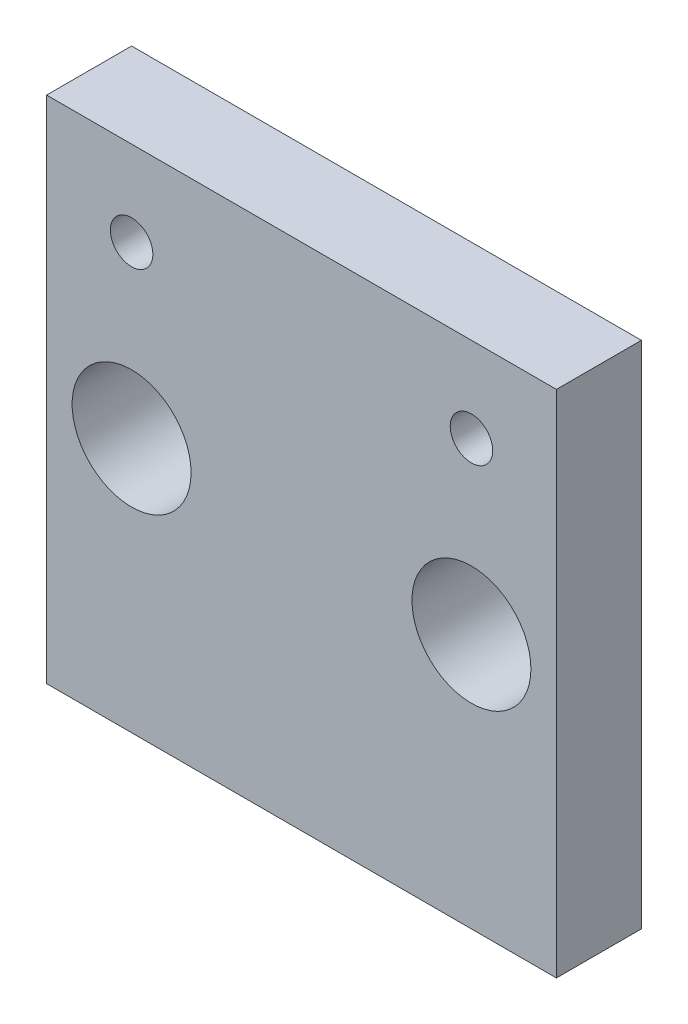
SolidWorks part; units mm, degrees
ref_plane "前视基准面" through (0, 0, 0) normal (0, 0, 1) x (1, 0, 0)
ref_plane "上视基准面" through (0, 0, 0) normal (0, 1, 0) x (1, 0, 0)
ref_plane "右视基准面" through (0, 0, 0) normal (1, 0, 0) x (0, 0, -1)
ref_plane "基准面4" through (0, 0, 5) normal (0, 0, 1) x (1, 0, 0)
sketch "草图1" plane through (0, 0, 5) normal (0, 0, 1) x (1, 0, 0)
  line L0 (-15, -15) -> (15, -15)
  line L1 (15, -15) -> (15, 15)
  line L2 (15, 15) -> (-15, 15)
  line L3 (-15, 15) -> (-15, -15)
  circle A2 centre (-10, 10) radius 1.25
  circle A3 centre (10, 10) radius 1.25
extrude "凸台-拉伸1" add sketch "草图1" against normal blind 5
hole_wizard "Ø7.0 (7) 直径孔1" positions "草图3" profile "草图4" hole size "Ø7.0" standard "GB" end condition through all
sketch "草图3" plane through (0, 0, 5) normal (0, 0, 1) x (1, 0, 0)
  line L0 (0, -15) -> (0, 4.8812) construction
  line L1 (-15, -15) -> (15, -15) construction
  point P0 (10, 0)
  point P2 (-10, 0)
  dimension "D1" = 20
  dimension "D2" = 15
sketch "草图4" plane through (10, 0, 5) normal (1, 0, 0) x (0, -1, 0)
  line L0 (0, 0) -> (0, 5)
  line L1 (0, 5) -> (3.5, 5)
  line L2 (3.5, 5) -> (3.5, 0)
  line L5 (3.5, 0) -> (0, 0)
  line L11 (0, -6.35) -> (0, 107.95) construction
  dimension "通孔孔直径" = 7
  dimension "通孔孔深度" = 5
